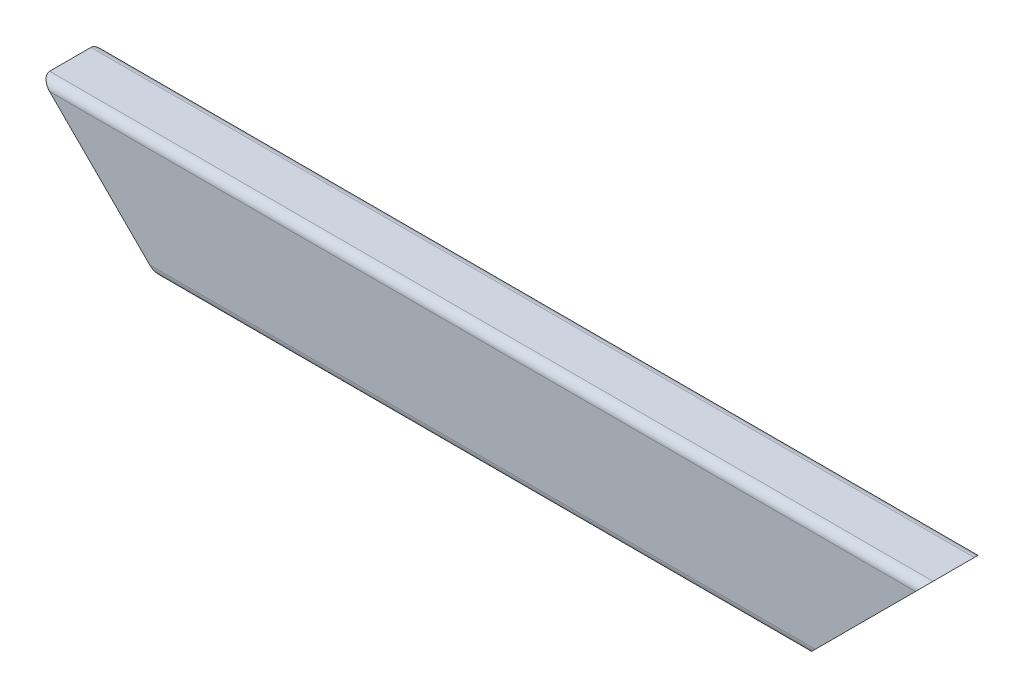
from build123d import *

# Parameters (mm, degrees)
COLD_FORMED_RECT_HOLLOW_SECTION_GB_T_672_DEPTH = 600
CUT_EXTRUDE1_DEPTH                             = 603.660766933


with BuildPart() as part:
    # Sketch1 → Cold-Formed Rect Hollow Section GB/T 6728-2002 80 X 40 X 3(1) (new body)
    with BuildSketch(Plane(origin=(0, 0, 0), x_dir=(0, 0, -1), z_dir=(1, 0, 0))):
        with BuildLine():
            Line((-14, -40), (14, -40))
            ThreePointArc((14, -40), (18.242640687, -38.242640687), (20, -34))
            Line((20, -34), (20, 34))
            ThreePointArc((20, 34), (18.242640687, 38.242640687), (14, 40))
            Line((14, 40), (-14, 40))
            ThreePointArc((-14, 40), (-18.242640687, 38.242640687), (-20, 34))
            Line((-20, 34), (-20, -34))
            ThreePointArc((-20, -34), (-18.242640687, -38.242640687), (-14, -40))
        make_face()
        with BuildLine():
            Line((-14, -37), (14, -37))
            ThreePointArc((14, -37), (16.121320344, -36.121320344), (17, -34))
            Line((17, -34), (17, 34))
            ThreePointArc((17, 34), (16.121320344, 36.121320344), (14, 37))
            Line((14, 37), (-14, 37))
            ThreePointArc((-14, 37), (-16.121320344, 36.121320344), (-17, 34))
            Line((-17, 34), (-17, -34))
            ThreePointArc((-17, -34), (-16.121320344, -36.121320344), (-14, -37))
        make_face(mode=Mode.SUBTRACT)
    extrude(amount=COLD_FORMED_RECT_HOLLOW_SECTION_GB_T_672_DEPTH)

    # Sketch2 → Cut-Extrude1 (cut, through all)
    with BuildSketch(Plane.XY.offset(20)):
        Polygon((74, -34), (6, 34), (0, 34), (0, -34), align=None)
        Polygon((600, 34), (594, 34), (526, -34), (600, -34), align=None)
        Polygon((600, -34), (526, -34), (520, -40), (600, -40), align=None)
        Polygon((6, 34), (0, 40), (0, 34), align=None)
        Polygon((600, 40), (594, 34), (600, 34), align=None)
        Polygon((80, -40), (74, -34), (0, -34), (0, -40), align=None)
    extrude(amount=-CUT_EXTRUDE1_DEPTH, mode=Mode.SUBTRACT)


solid = part.part
